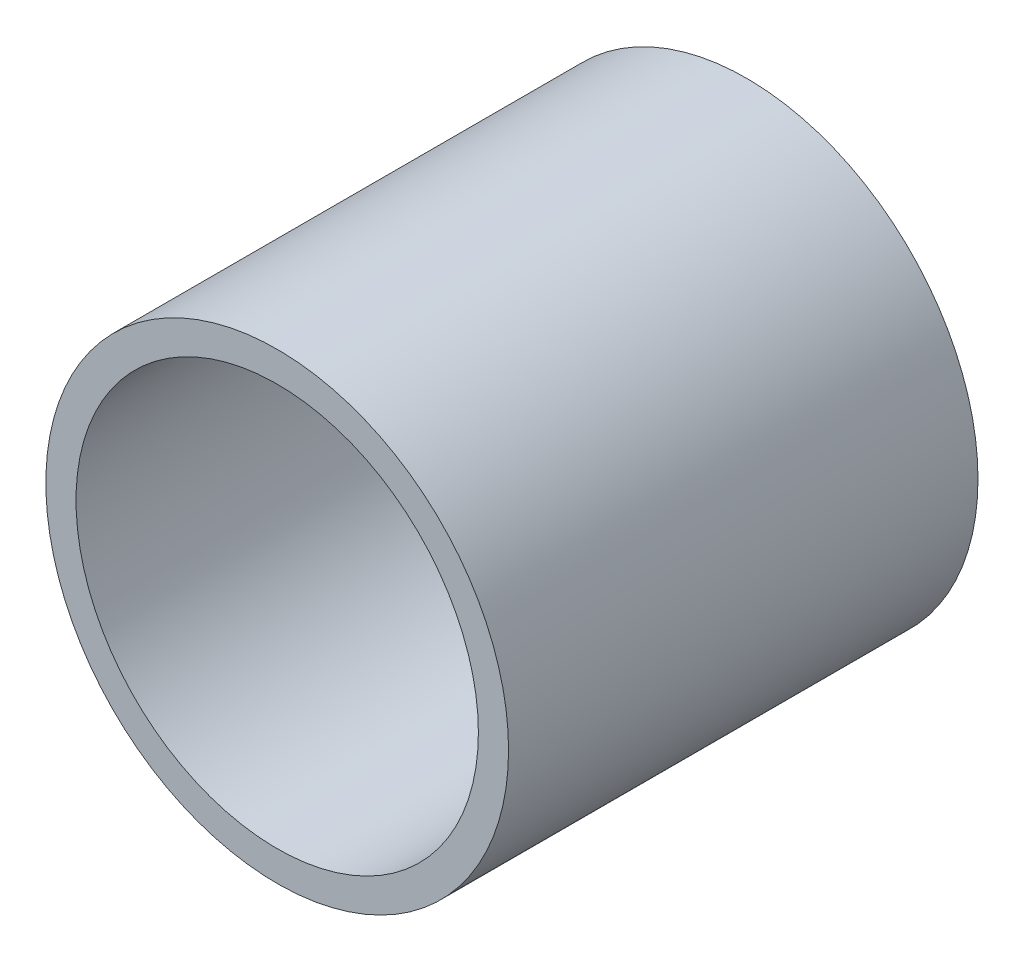
SolidWorks part; units mm, degrees
ref_plane "Front Plane" through (0, 0, 0) normal (0, 0, 1) x (1, 0, 0)
ref_plane "Top Plane" through (0, 0, 0) normal (0, 1, 0) x (1, 0, 0)
ref_plane "Right Plane" through (0, 0, 0) normal (1, 0, 0) x (0, 0, -1)
sketch "Sketch1" plane through (0, 0, 0) normal (0, 0, 1) x (1, 0, 0)
  circle A2 centre (0, 0) radius 3.45
  circle A3 centre (0, 0) radius 3.45 construction
  circle A4 centre (0, 0) radius 3.45 construction
  circle A5 centre (0, 0) radius 3
extrude "Boss-Extrude1" add sketch "Sketch1" along normal blind 7
